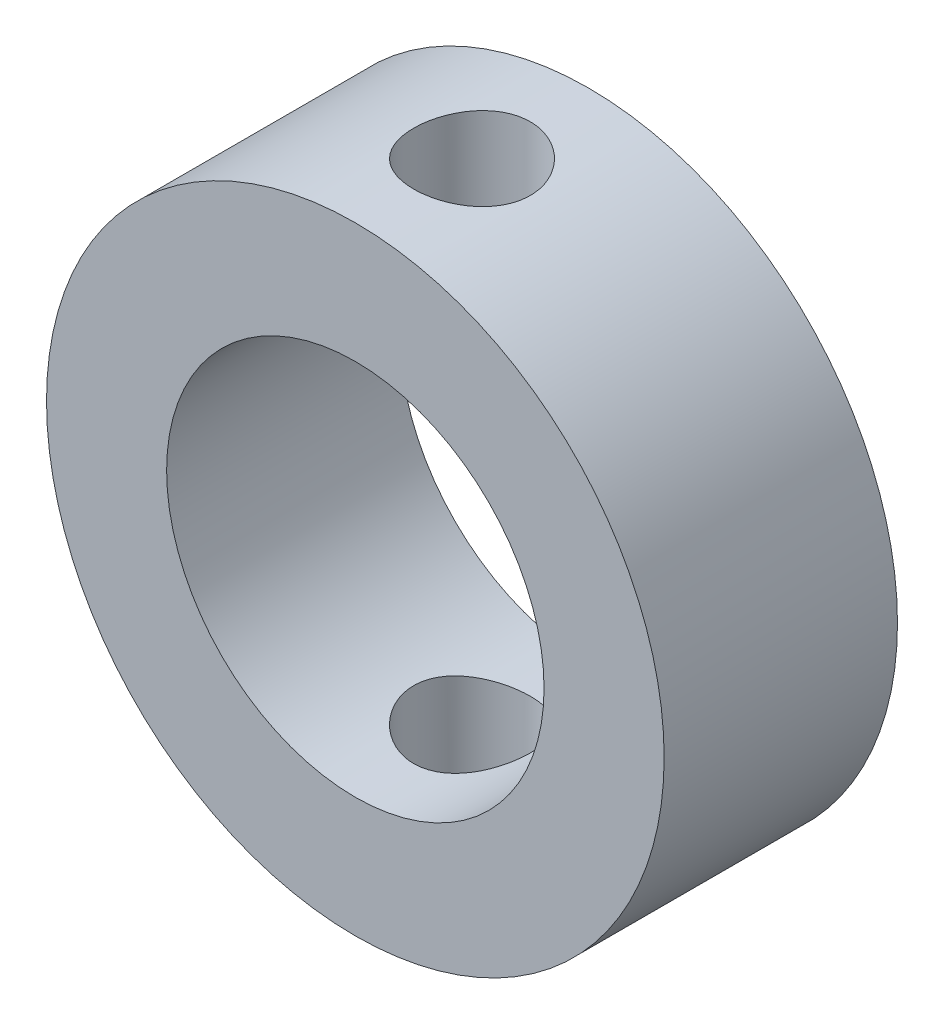
from build123d import *

# Parameters (mm, degrees)
SKETCH2_R               = 45
SKETCH2_R_2             = 27.5
BOSS_EXTRUDE1_DEPTH     = 34
CUT_EXTRUDE1_DEPTH      = 73.15261603
CUT_EXTRUDE1_DEPTH_BACK = 73.15261603
SKETCH3_R               = 8.5


with BuildPart() as part:
    # Sketch2 → Boss-Extrude1 (new body)
    with BuildSketch(Plane.XY):
        Circle(SKETCH2_R)
        Circle(SKETCH2_R_2, mode=Mode.SUBTRACT)
    extrude(amount=BOSS_EXTRUDE1_DEPTH)

    # Sketch3 → Cut-Extrude1 (cut, two sides: drawn at the far end of the back side and taken through both)
    with BuildSketch(Plane(origin=(0, 0, 0), x_dir=(1, 0, 0), z_dir=(0, 1, 0)).offset(-CUT_EXTRUDE1_DEPTH_BACK)):
        with Locations(Location((0, -17, 0), (0, 0, 270))):
            Circle(SKETCH3_R)
    extrude(amount=CUT_EXTRUDE1_DEPTH + CUT_EXTRUDE1_DEPTH_BACK, mode=Mode.SUBTRACT)


solid = part.part
